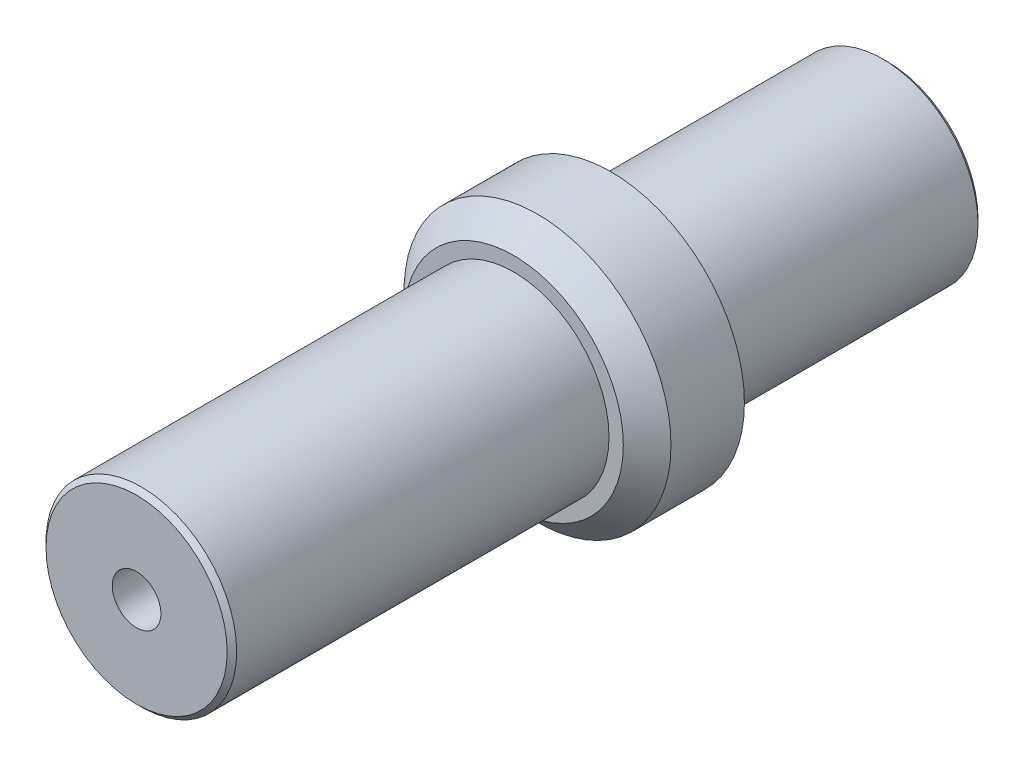
SolidWorks part; units mm, degrees
material "1023 碳钢板 (SS)"
ref_plane "前视基准面" through (0, 0, 0) normal (0, 0, 1) x (1, 0, 0)
ref_plane "上视基准面" through (0, 0, 0) normal (0, 1, 0) x (1, 0, 0)
ref_plane "右视基准面" through (0, 0, 0) normal (1, 0, 0) x (0, 0, -1)
sketch "草图1" plane through (0, 0, 0) normal (0, 0, 1) x (1, 0, 0)
  circle A0 centre (0, 0) radius 20
  dimension "D1" = 40
extrude "凸台-拉伸1" add sketch "草图1" along normal blind 58
sketch "草图2" plane through (0, 0, 58) normal (0, 0, 1) x (1, 0, 0)
  circle A0 centre (0, 0) radius 28
  dimension "D1" = 56
extrude "凸台-拉伸2" add sketch "草图2" along normal blind 20.4
sketch "草图3" plane through (0, 0, 78.4) normal (0, 0, 1) x (1, 0, 0)
  circle A0 centre (0, 0) radius 20
  dimension "D1" = 40
extrude "凸台-拉伸3" add sketch "草图3" along normal blind 79.1
chamfer "倒角1" distance 5 angle 45 1 edges at (28, 0, 78.4)
chamfer "倒角2" distance 1 angle 45 2 edges at (20, 0, 157.5) (20, 0, 0)
hole_wizard "M12 螺纹孔1" positions "草图4" profile "草图5" tap size "M12" standard "ISO"
sketch "草图4" plane through (0, 0, 0) normal (0, 0, -1) x (-1, 0, 0)
  point P0 (0, 0)
sketch "草图5" plane through (0, 0, 0) normal (1, 0, 0) x (0, 1, 0)
  line L0 (0, 0) -> (0, 32.3144)
  line L1 (0, 32.3144) -> (5.1, 29.25)
  line L2 (5.1, 29.25) -> (5.1, 0)
  line L5 (5.1, 0) -> (0, 0)
  line L10 (0, 32.3144) -> (-5.1, 29.25) construction
  line L11 (0, -6.35) -> (0, 107.95) construction
  dimension "螺纹孔钻头直径" = 10.2
  dimension "螺纹孔钻头深度" = 29.25
  dimension "导头角度" = 118
cosmetic thread "孔螺蚊线1" parameters "D1"=24, "D2"=12
hole_wizard "M12 螺纹孔2" positions "草图6" profile "草图7" tap size "M12" standard "ISO"
sketch "草图6" plane through (0, 0, 157.5) normal (0, 0, 1) x (1, 0, 0)
  point P0 (0, 0)
sketch "草图7" plane through (0, 0, 157.5) normal (1, 0, 0) x (0, -1, 0)
  line L0 (0, 0) -> (0, 32.3144)
  line L1 (0, 32.3144) -> (5.1, 29.25)
  line L2 (5.1, 29.25) -> (5.1, 0)
  line L5 (5.1, 0) -> (0, 0)
  line L10 (0, 32.3144) -> (-5.1, 29.25) construction
  line L11 (0, -6.35) -> (0, 107.95) construction
  dimension "螺纹孔钻头直径" = 10.2
  dimension "螺纹孔钻头深度" = 29.25
  dimension "导头角度" = 118
cosmetic thread "孔螺蚊线2" parameters "D1"=24, "D2"=12
